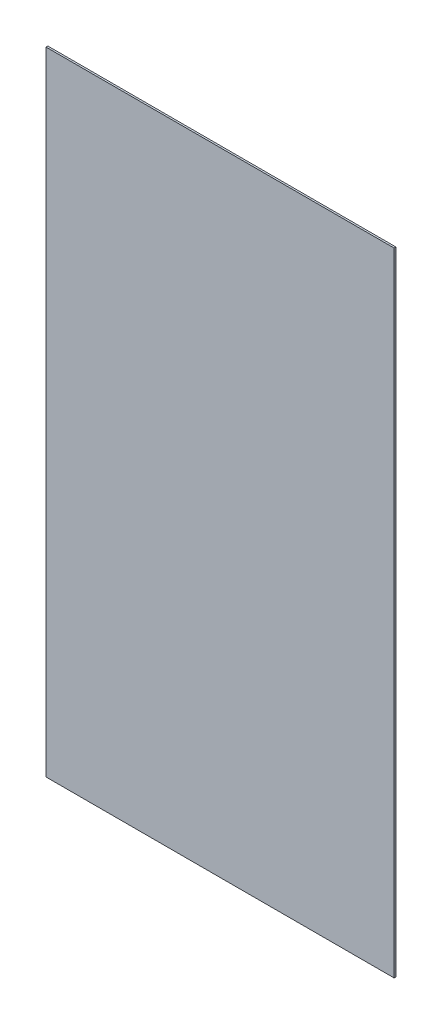
from build123d import *

# Parameters (mm, degrees)
SKETCH_1_W      = 380
SKETCH_1_H      = 690
EXTRUDE_1_DEPTH = 2


with BuildPart() as part:
    # 草图1 → 凸台-拉伸1 (new body)
    with BuildSketch(Plane.XY):
        with Locations((-147.881773399, -183.54679803)):
            Rectangle(SKETCH_1_W, SKETCH_1_H)
    extrude(amount=EXTRUDE_1_DEPTH)


solid = part.part
